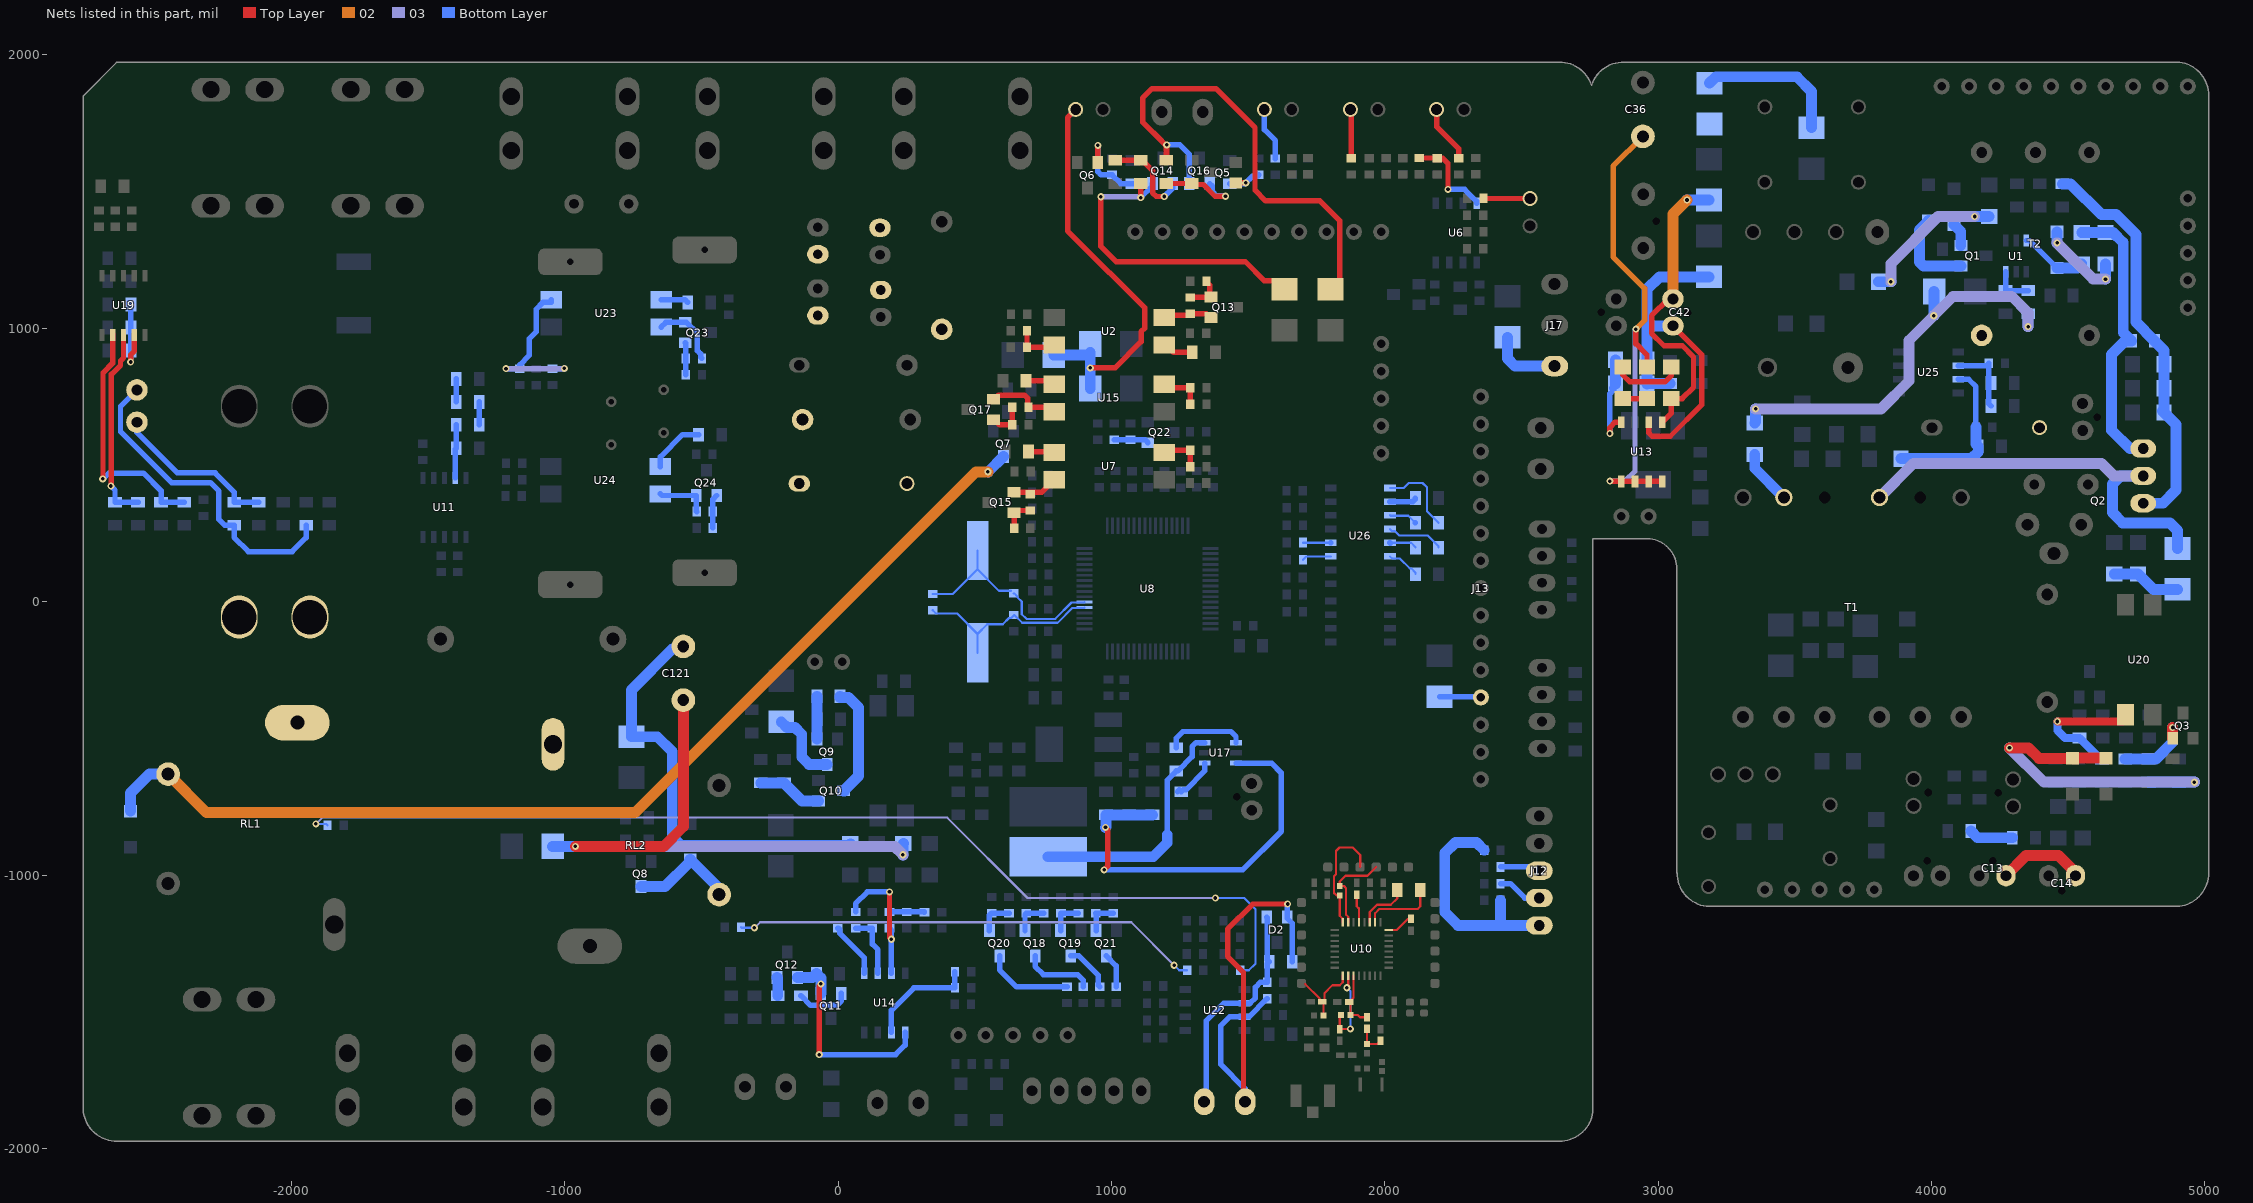
[diagram p0: the nets of this part, all layers, seen from the top]
# Altium PCB MISC105418.PcbDoc (part 5 of 7)
Units mil, origin at the board's own origin, x right, y up, seen from the top; angles counter-clockwise.
Board outline 7774.32 x 3947.04 mil, 4 copper layers (Top Layer, 02, 03, Bottom Layer), stack 30.635 mil thick; 459 components, 285 nets, 1258 pads, 468 vias.
Unrouted connection lines stored in the file: 23.

## Via types
v1: diameter 26, hole 13, Top Layer to Bottom Layer, tented both sides, 468 vias

## Nets (pads, with @x,y where several pads share a name; then routed paths per layer and width w, separated by ;. In a path a pad name is that pad's centre, name@x,y a point inside that pad or via, vN(x,y) a via of type N, cw(c..) or ccw(c..) an arc to the next point about the centre after c; other vN are vias at no path point) (continued)
NetC13_2: C13.2 C14.1 | length 321.8
  Top Layer w40: C13.2@4272.11,-1002.49 4345.61,-929 4464.5,-929 4526.11,-990.61 C14.1@4526.11,-1002.49
NetC17_2: C17.2 U26.2 | length 100.9
  Bottom Layer w20: U26.2@2018.36,365.7 2101.99,365.7 2111.68,375.39 C17.2@2111.68,379
NetC18_1: C18.1 U26.3 | length 106.4
  Bottom Layer w8: U26.3@2018.36,315.7 2020.06,314 2085.8,314 C18.1@2111.68,288.12
  Bottom Layer w20: C18.1@2110.51,289.29 C18.1@2111.68,288.12
NetC18_2: C18.2 U26.1 | length 297.3
  Bottom Layer w8: U26.1@2018.36,415.7 2068.7,415.7 2087,434 2138,434 2154,418 2154,330.44 C18.2@2196.32,288.12
NetC19_1: C19.1 U26.5 | length 95.2
  Bottom Layer w8: U26.5@2027.81,215.7 2095.99,215.7 2111.68,200.02 C19.1@2111.68,197.52
  Bottom Layer w20: U26.5@2018.36,215.7 U26.5@2020.04,214.03
NetC19_2: C19.2 U26.4 | length 209.3
  Bottom Layer w8: U26.4@2018.36,265.7 2026.06,258 2037,258 2053,242 2157.16,242 2196.32,202.83 C19.2@2196.32,197.52
NetC23_2: C23.2 U26.6 | length 123.4
  Bottom Layer w8: U26.6@2018.36,165.7 2026.56,157.5 2054.97,157.5 2090.77,121.7 2096.09,121.7 2111.77,106.02 C23.2@2111.77,100.7
NetC27_1: C27.1 U17.1 | length 293.8
  Bottom Layer w20: C27.1@1237.09,-534.64 1237.09,-498.91 1261,-475 1437,-475 1455.48,-493.48 U17.1@1455.48,-515.6
NetC27_2: C27.2 L29.1 U17.6 | length 902
  Bottom Layer w20: 1204,-853 1204,-652.38 C27.2@1237.09,-619.29 1242.71,-619.29 1295,-567 1295,-530 1309.4,-515.6 U17.6@1340.91,-515.6
  Bottom Layer w39.37: L29.1@768,-933.03 1152.97,-933.03 1204,-882 1204,-853
NetC33_2: C33.2 R36.2 R37.1 U17.3 | length 1481.4
  Top Layer w20: v1(973,-981) 986,-968 986,-834 v1(978,-826)
  Bottom Layer w20: v1(973,-981) 1480,-981 1621,-840 1621,-626 1585.4,-590.4 U17.3@1455.48,-590.4
  Bottom Layer w40: v1(978,-826) 980.08,-823.92 C33.2@980.08,-779.82 R36.2@1065.08,-779.82 R37.1@1150.08,-779.82
NetC36_1: C36.1 D3.2 R92.2 U13.5 U13.6 U13.7 U13.8 | length 1788.1
  Top Layer w19.68: v1(2823,441) 2824.27,439.73 U13.5@2865,439.73 U13.6@2915,439.73 U13.7@2965,439.73 U13.8@3015,439.73 ; v1(2918,997) 2918,944 2959,903 R92.2@2959,857.56
  02 w19.68: v1(2918,997) 2950,1029 2950,1146 2835,1261 2835,1593 C36.1@2944,1702
  03 w19.68: v1(2823,441) 2879,441 2915,477 2915,994 v1(2918,997)
NetC38_2: C38.2 U10.8 | length 99.5
  Top Layer w8: U10.8@2013.52,-1201.6 2042.4,-1201.6 2083.46,-1160.54 C38.2@2096,-1160.54
NetC39_2: C39.2 R44.2 U8.6 Y1.1 | length 777.4
  Bottom Layer w8: R44.2@346,27.72 419.61,27.72 Y1.1@510,118.11 ; Y1.1@510,187.01 Y1.1@510,118.11 ; C39.2@632.28,40 588.11,40 Y1.1@510,118.11 ; C39.2@642,30.28 644.56,30.28 655.72,19.12 655.72,16.56 672,0.28 672,-46 689,-63 794,-63 853.98,-3.02 900.46,-3.02 U8.6@901.78,-1.71
NetC42_1: C42.1 D9.2 R39.1 U13.1 | length 1130
  Top Layer w19.68: U13.1@3015,656.27 3048,689.27 R39.1@3048,742.44 3087.44,742.44 3129,784 3129,895 3088,936 3021,936 2976,981 2976,1046 3037.02,1107.02 C42.1@3053.8,1107.02
  02 w39.37: C42.1@3053.8,1107.02 3053.8,1417.8 v1(3105.2,1469.2)
  Bottom Layer w39.37: v1(3105.2,1469.2) D9.2@3186,1469.2
NetC42_2: C42.2 D4.2 L1.1 R45.1 R88.1 U13.2 | length 1391.7
  Top Layer w19.68: U13.2@2965,656.27 2965,618 2978,605 3044,605 3159,720 3159,904.18 C42.2@3054.2,1008.98
  Bottom Layer w40: L1.1@3042.88,797.79 2960.71,797.79 R88.1@2959.42,796.5 R45.1@2959.42,884.55 2959.42,1017 ; C42.2@3054.2,1008.98 2967.44,1008.98 2959.42,1017 ; D4.2@3186,1188 3004,1188 2959.42,1143.42 2959.42,1017
NetC59_1: C59.1 C63.2 L11.2 | length 108.7
  Top Layer w8: C59.1@1935.09,-1563.03 L11.2@1935.09,-1617.95 1972.63,-1617.95 C63.2@1984.09,-1606.49
NetC59_2: C59.2 C61.2 L21.2 U10.27 | length 216
  Top Layer w8: U10.27@1885.57,-1368.92 1885.57,-1449.02 C61.2@1869.55,-1465.03 1873.97,-1469.45 L21.2@1873.97,-1512.03 1901.03,-1512.03 1909,-1520 1934.98,-1520 C59.2@1935.09,-1520.11
NetC60_2: C60.2 L21.1 U10.26 | length 294.3
  Top Layer w8: L21.1@1839.89,-1512.03 1835.09,-1516.83 C60.2@1835.09,-1563.57 1873.52,-1563.57 v1(1874.09,-1563) ; v1(1861,-1412.5) 1865.88,-1407.61 U10.26@1865.88,-1368.92
  Bottom Layer w8: v1(1861,-1412.5) 1874.09,-1425.59 v1(1874.09,-1563)
NetC79_2: C79.2 C80.1 | length 162.1
  Bottom Layer w40: C80.1@4143.42,-839.18 4167.99,-863.75 C79.2@4295.38,-863.75
NetC82_1: C82.1 Q3.1 R32.1 | length 292.5
  Top Layer w40: Q3.1@4881.69,-499.76 v1(4881.69,-460.31)
  Bottom Layer w40: C82.1@4708.09,-575.85 R32.1@4793.09,-575.85 ; R32.1@4793.09,-575.68 4820.32,-575.68 4881.69,-514.31 v1(4881.69,-460.31)
NetC89_1: C89.1 R181.1 U6.4 | length 338.1
  Top Layer w20: C89.1@2126,1622.91 2190.82,1622.91 R181.1@2192,1621.72 2212.28,1621.72 2231,1603 v1(2231,1508)
  Bottom Layer w20: v1(2231,1508) 2292.08,1508 2336.09,1463.98 U6.4@2336.09,1457.5
NetC98_1: C98.1 R182.2 U19.2 | length 916.8
  Top Layer w20: v1(-2690,449) -2690,451 -2689,452 -2689,837 -2653.37,872.63 U19.2@-2653.37,975.73
  Bottom Layer w20: v1(-2690,449) -2688.38,449 -2667.38,470 -2541,470 -2476.66,405.66 R182.2@-2476.66,363.96 C98.1@-2392.18,363.96
NetC99_2: C99.2 R184.2 U19.3 | length 721.2
  Top Layer w20: v1(-2660,423) -2658,425 -2658,831 -2625,864 -2625,880.64 -2614,891.64 -2614,913.4 U19.3@-2614,975.73
  Bottom Layer w20: v1(-2660,423) -2645.15,408.15 R184.2@-2645.15,363.96 C99.2@-2560.91,363.96
NetC100_1: C100.1 R187.1 R188.1 U19.4 | length 315.6
  Top Layer w20: v1(-2588,876.62) -2588,902.63 -2574.63,916 U19.4@-2574.63,975.73
  Bottom Layer w20: v1(-2588,876.62) -2586.91,877.72 R187.1@-2586.91,918.67 C100.1@-2586.91,1002.7 R188.1@-2586.91,1087.17
NetC101_1: C101.1 U10.13 | length 104
  Top Layer w8: C101.1@1897,-1071.49 1897,-1114 1905.25,-1122.25 U10.13@1905.25,-1172.07
NetC110_1: C110.1 R44.1 U8.5 Y1.2 | length 724.1
  Bottom Layer w8: R44.1@346,-31.72 357.16,-42.88 434.77,-42.88 Y1.2@510,-118.11 ; Y1.2@510,-187.01 Y1.2@510,-118.11 ; U8.5@901.84,-21.45 900.58,-22.71 857.29,-22.71 803,-77 673.01,-77 644.56,-48.55 633.4,-59.71 625.29,-59.71 602.26,-82.74 545.37,-82.74 Y1.2@510,-118.11
NetC114_1: C114.1 R81.1 R82.2 | length 127.9
  Bottom Layer w20: R81.1@188.3,-1134.98 R82.2@251.44,-1134.98 314.57,-1134.98 C114.1@315.76,-1136.16
NetC119_1: C119.1 R193.1 R194.2 U25.2 | length 275.2
  Bottom Layer w19.68: U25.2@4097.36,863.5 4200.55,863.5 C119.1@4209.05,872 4209.05,724.05 R194.2@4217.57,715.53
NetC120_2: C120.2 R191.1 R192.2 U25.3 | length 610.6
  Bottom Layer w19.68: U25.3@4097.36,813.5 4135.5,813.5 4162.05,786.95 C120.2@4162.05,638.5
  Bottom Layer w40: R191.1@3888.56,523.35 4146.35,523.35 4170.57,547.57 R192.2@4170.57,568.5 4162.05,577.03 C120.2@4162.05,638.5
NetC121_1: C121.1 D29.2 R263.2 | length 2235.2
  Top Layer w40: v1(-961,-895) -638,-895 -566.28,-823.28 -566.28,-500.28 C121.1@-566.28,-360.31
  03 w40: v1(-961,-895) 206,-895 v1(237,-926)
  Bottom Layer w40: D29.2@-1044.2,-895 v1(-961,-895) ; C121.1@-566.28,-360.31 C121.1@-566.28,-347.7 ; v1(237,-926) 237,-886.87 R263.2@238.43,-885.44
NetC121_2: C121.2 D30.1 R200.2 | length 1577.5
  Bottom Layer w39.37: C121.2@-566.28,-163.47 -575.32,-172.5 -605.5,-172.5 -756,-323 D30.1@-756,-493.77 -661.23,-493.77 -607,-548 -607,-859 -574,-892 38.54,-892 R200.2@45.09,-885.44
NetC129_1: C129.1 R42.2 U10.25 | length 283.8
  Top Layer w8: 1709,-1399 1761,-1451 1761,-1453.4 C129.1@1771.17,-1463.58 ; R42.2@1775.59,-1513.58 1775.59,-1467.99 C129.1@1771.17,-1463.58 ; U10.25@1846.2,-1368.92 1846.2,-1392.02 1835.22,-1403 1808,-1403 1779,-1432 1779,-1455.75 C129.1@1771.17,-1463.58
NetCX1_1: CX1.1 L28.2 L30.1 Y2.1
NetCX1_2: CX1.2 L26.2 L27.1 Y3.2
NetCX3_1: CX3.1 T2.4
NetD2_1: D2.1 J7.1 R176.1 R178.2 U22.6 | length 847.9
  Bottom Layer w19.68: D2.1@1567.8,-1154.24 1569.67,-1156.11 1569.67,-1310.15 R176.1@1576.65,-1317.14
  Bottom Layer w20: J7.1@1338.98,-1829.5 1346.45,-1822.02 1346.45,-1533.55 1411.04,-1468.96 U22.6@1486.06,-1468.96 1507.04,-1468.96 1526,-1450 1526,-1411 1544.86,-1392.14 R178.2@1569.31,-1392.14 1569.31,-1324.48 R176.1@1576.65,-1317.14
NetD2_2: D2.2 J7.2 R171.1 R176.2 U22.7 | length 1661
  Top Layer w19.68: J7.2@1488.98,-1829.5 1483,-1823.52 1483,-1356 1425,-1298 1425,-1198 1517,-1106 v1(1644,-1106)
  Bottom Layer w19.68: v1(1644,-1106) 1642.6,-1107.4 D2.2@1642.6,-1154.24 1642.6,-1158.17 1661.3,-1176.87 R176.2@1661.3,-1317.14
  Bottom Layer w20: J7.2@1488.98,-1829.5 1488.98,-1781.98 1399,-1692 1399,-1552 1432.04,-1518.96 U22.7@1486.06,-1518.96 1502.49,-1518.96 R171.1@1569.31,-1452.14
NetD3_1: D3.1 D11.2 | length 537.1
  Bottom Layer w40: D3.1@3188,1896.8 3211.2,1920 3506.8,1920 3561,1865.8 D11.2@3561,1733.8
NetD6_2: D6.2 D10.2 D19.2 J25.2 | length 1480
  Top Layer w20: J25.2@869.09,1800.5 839.17,1770.58 839.17,1356.54 993.56,1202.16 994.84,1202.16 1122,1075 1122,1000.77 1108.78,987.55 1108.78,950.78 1013,855 v1(922.2,855)
  Bottom Layer w40: D19.2@788.8,901.67 912.86,901.67 922.2,911 v1(922.2,855) D10.2@922.2,780
NetD7_2: D7.2 J17.1 | length 262.3
  Bottom Layer w40: D7.2@2448.09,966.9 2448.09,888.91 2475.3,861.7 J17.1@2621.09,861.7
NetD8_2: D8.2 Q14.2 R129.1 | length 1186.6
  Top Layer w19.68: v1(961,1481) 961,1299.71 1017,1243.71 1489.29,1243.71 1558.7,1174.3 1601.5,1174.3 D8.2@1633,1142.8 ; v1(1107,1478) 1107.13,1478.13 1107.13,1529.55 R129.1@1107.26,1529.68
  03 w19.68: v1(961,1481) 1104,1481 v1(1107,1478)
  Bottom Layer w19.68: v1(1107,1478) 1149.69,1520.69 Q14.2@1149.69,1529.62
NetD12_1: D12.1 Q7.3 RL1.2 | length 3885.7
  02 w40: RL1.2@-2450.87,-631 -2309.87,-772 -743,-772 504,475 v1(548,475)
  Bottom Layer w40: D12.1@-2588,-766.06 -2588,-700 -2519,-631 RL1.2@-2450.87,-631 ; v1(548,475) 549.26,475 Q7.3@605,530.74
NetD13_1: D13.1 Q8.3 RL2.2 | length 393.9
  Bottom Layer w40: Q8.3@-721.34,-1042.41 -633.41,-1042.41 -544.62,-953.62 -544.62,-946.58 -541.98,-943.94 D13.1@-540.02,-943.94 ; D13.1@-537.38,-946.58 -444.13,-1039.83 -444.13,-1063.03 RL2.2@-435.21,-1071.94
NetD14_1: D14.1 Q9.3 | length 281.1
  Bottom Layer w40: D14.1@-207.91,-439.47 -186.57,-460.81 -157.19,-460.81 -133,-485 -133,-568 -105.74,-595.26 Q9.3@-40,-595.26
NetD16_2: D16.2 Q16.2 R135.1 | length 1862.1
  Top Layer w20: v1@1199.57,1668.57 1200.26,1667.87 R135.1@1200.26,1614.32 1202,1616.06 v1(1202,1671) 1197.13,1671 1171.07,1697.06 1130.07,1738.07 1114,1754.13 1114,1842 1149,1877 1382.28,1877 1525,1734.28 1525,1505 1564,1466 1762,1466 1835,1393 1835,1174.14 1803.66,1142.8 D16.2@1801,1142.8
  Bottom Layer w20: v1(1202,1671) 1250,1671 1284.69,1636.31 Q16.2@1284.69,1529.62
NetD20_1: D20.1 Q1.2 | length 85.9
  Bottom Layer w39.37: D20.1@4082.09,1378.54 4106.83,1353.8 Q1.2@4106.83,1302.91
NetD21_1: D21.1 R12.1 | length 327.8
  03 w40: v1(4459.09,1312.09) 4591.09,1180.09 v1(4636.09,1180.09)
  Bottom Layer w40: v1@4459,1312 v1(4459.09,1312.09) D21.1@4459.09,1352.39 ; v1(4636.09,1180.09) R12.1@4636.09,1235.78
NetD21_2: D21.2 R10.1 U1.6 | length 250.7
  Bottom Layer w19.68: U1.6@4346.4,1321.09 4358.51,1321.09 D21.2@4459.09,1220.5
  Bottom Layer w39.37: D21.2@4459.09,1220.5 4533.82,1220.5 R10.1@4549.09,1235.78
NetD22_1: D22.1 R6.1 R20.1 | length 1519.1
  03 w40: v1(3356,705) 3815,705 3918,808 3918,956 v1(4008,1046) 4079,1117 4293,1117 4353,1057 v1(4353,1006)
  Bottom Layer w40: R20.1@3353,653.56 3356,656.56 v1(3356,705) ; v1(4008,1046) 4009.29,1047.29 D22.1@4009.29,1134.5 ; v1(4353,1006) 4353.09,1006.09 R6.1@4353.09,1053.18
NetD23_1: D23.1 Q2.2 T1.3 | length 1595.7
  03 w40: T1.3@3809.09,381.08 3933.02,505 4622,505 4667.03,459.97 Q2.2@4773.87,459.97
  Bottom Layer w40: Q2.2@4773.87,459.97 4690.97,459.97 4661,430 4661,326 4699,288 4872,288 4899.09,260.91 D23.1@4899.09,194.31
NetD23_2: D23.2 R17.1 R19.1 | length 254.5
  Bottom Layer w40: R17.1@4668.09,101.32 R19.1@4755.09,101.32 4811.71,44.7 D23.2@4899.09,44.7
NetD555_2: D555.2 J13.12 | length 151.9
  Bottom Layer w20: D555.2@2200.09,-348.1 2348.9,-348.1 J13.12@2351.09,-350.3
NetJ1_2: J1.2 R113.2 | length 212.3
  Top Layer w20: J1.2@2189.09,1800.5 2189.09,1737.91 2270,1657 R113.2@2270,1621.72
NetJ2_2: J2.2 R114.2 | length 170.5
  Top Layer w20: R114.2@2361.09,1476 2362.39,1474.7 J2.2@2531.09,1474.7
NetJ3_2: J3.2 R121.1 | length 180
  Top Layer w20: J3.2@1874.09,1800.5 1877,1797.6 R121.1@1877,1621.72
NetJ4_2: J4.2 R122.1 | length 196.4
  Bottom Layer w20: J4.2@1559.09,1800.5 1559.09,1726.91 1599.09,1686.91 R122.1@1599.09,1620.69
NetJ12_1: J12.1 R233.2 R234.1 | length 848.4
  Bottom Layer w40: R233.2@2363.65,-909.5 2335.15,-881 2258,-881 2219,-920 2219,-1135 2268.3,-1184.3 2559.09,-1184.3 J12.1@2565.09,-1190.3 ; 2423.09,-1184.3 R234.1@2423.09,-1092.5
NetJ12_2: J12.2 R235.1 | length 163.9
  Bottom Layer w20: R235.1@2423.09,-1031.5 2459.5,-1031.5 2512.3,-1084.3 J12.2@2565.09,-1084.3
NetJ12_3: J12.3 R236.1 | length 147.7
  Bottom Layer w20: R236.1@2423.09,-970.5 2551.29,-970.5 J12.3@2565.09,-984.3
NetJP1_2: pad.1@-2191,-56.5 RL1.1
NetJP2_2: pad.1@-1932,-56.5 RL2.4
NetL22_1: L22.1 U10.10 | length 267.6
  Top Layer w8: U10.10@1964.31,-1172.07 1964.31,-1139.69 1980,-1124 2120,-1124 2129.65,-1114.35 L22.1@2129.65,-1055
NetL22_2: L22.2 U10.11 | length 188.5
  Top Layer w8: U10.11@1944.62,-1172.07 1944.62,-1135.38 1971,-1109 2022,-1109 2045,-1086 L22.2@2045,-1055
NetQ1_1: Q1.1 R11.2 ZD1.2 | length 322.2
  Bottom Layer w40: ZD1.2@3989.09,1393.5 3955.57,1359.98 R11.2@3955.57,1289.13 3955.57,1242.43 3969.9,1228.1 Q1.1@4106.83,1228.1
NetQ2_1: Q2.1 R10.2 R12.2 R15.1 | length 1053.4
  Bottom Layer w40: R10.2@4549.09,1350.9 R12.2@4636.09,1350.9 4663.1,1350.9 4701,1313 4701,983.99 R15.1@4730.99,954 4708,954 4658,904 4658,627 4725.03,559.97 Q2.1@4773.87,559.97
NetQ2_3: Q2.3 R9.2 R13.1 R15.2 R16.1 R241.1 | length 1489
  Bottom Layer w40: R9.2@4478.09,1528.35 4508.65,1528.35 4621,1416 4674,1416 4747,1343 4747,1022.64 R15.2@4815.64,954 4850.56,919.08 R16.1@4850.56,869 R13.1@4850.56,780.5 R241.1@4850.56,692 ; Q2.3@4773.87,359.97 4845.97,359.97 4894,408 4894,648.56 R241.1@4850.56,692 ; R241.1@4845.34,697.22 R241.1@4850.56,692
NetQ5_1: Q5.1 R56.2 R58.2 | length 152.5
  Top Layer w20: Q5.1@1454.52,1531.6 1454.72,1531.8 1490.8,1531.8 v1(1491,1532)
  Bottom Layer w20: R58.2@1432.09,1528.7 v1@1487.7,1528.7 ; v1(1491,1532) 1515.08,1556.08 1533.94,1556.08 R56.2@1539.09,1561.24
NetQ6_1: Q6.1 R57.1 R59.2 | length 304.4
  Top Layer w20: Q6.1@949.66,1606.34 949.83,1606.51 949.83,1668.83 v1(950,1669)
  Bottom Layer w20: v1(950,1669) 949.83,1668.83 949.83,1573.12 961.72,1561.24 R57.1@1002.09,1561.24 1034.63,1528.7 R59.2@1077.09,1528.7
NetQ9_1: Q9.1 R69.2 R70.2 | length 156.8
  Bottom Layer w40: Q9.1@-77.4,-502.74 Q9.1@-77.4,-502.74 -77.36,-346.04 R69.2@-77.32,-346
NetQ10_1: Q10.1 R72.2 R73.2 | length 238
  Bottom Layer w40: R73.2@-282.91,-663.44 -197.91,-663.44 -131.94,-729.4 Q10.1@-72.26,-729.4
NetQ10_3: Q10.3 R69.1 | length 416.6
  Bottom Layer w40: R69.1@7.32,-346 7.32,-350.69 7.64,-351 38.25,-351 75,-387.75 75,-637.26 23.88,-688.38 23.88,-691.69 23.57,-692 Q10.3@20.26,-692
NetQ11_1: Q11.1 Q12.1 R75.2 U14.1 | length 789.6
  Top Layer w20: v1(-69,-1657) -69,-1405.54 -63.31,-1399.84 v1(-63.31,-1398.22)
  Bottom Layer w20: v1(-69,-1657) 210.55,-1657 245.09,-1622.46 U14.1@245.09,-1575.76
  Bottom Layer w40: Q12.1@-148.5,-1374.54 -93.04,-1374.54 R75.2@-79.32,-1360.82 -63.31,-1376.83 v1(-63.31,-1398.22) Q11.1@-63.31,-1432.7
NetQ11_2: Q11.2 R97.1 | length 196.7
  Bottom Layer w20: R97.1@-135.91,-1441.5 -100.4,-1477 -5,-1477 11.5,-1460.5 Q11.2@11.5,-1432.7
NetQ12_2: Q12.2 R99.2 | length 68
  Bottom Layer w40: Q12.2@-223.31,-1374.54 -220.91,-1376.94 R99.2@-220.91,-1441.5
NetQ13_1: Q13.1 R64.1 R65.2 | length 140.7
  Top Layer w20: R64.1@1288.58,1112.79 1289.34,1113.55 1363.47,1113.55 Q13.1@1364.23,1114.31 1360.29,1118.24 1360.29,1156.89 1347.83,1169.35 R65.2@1347.83,1171.91
NetQ13_2: Q13.2 R64.2 U2.2 | length 183.1
  Top Layer w20: U2.2@1192.79,1038.91 1202.07,1048.18 1283.42,1048.18 R64.2@1288.58,1053.34 1346.45,1053.34 1360.29,1039.5 Q13.2@1364.23,1039.5
NetQ14_1: Q14.1 R129.2 R130.2 | length 341.6
  Top Layer w20: R130.2@1014.26,1614.32 1112.57,1614.32 1150.54,1576.35 1150.54,1495.46 1164,1482 v1(1193,1482)
  Bottom Layer w20: v1(1193,1482) 1224.5,1513.5 Q14.1@1224.5,1529.62
NetQ15_1: Q15.1 R80.1 R85.1 | length 120
  Top Layer w19.68: R85.1@643.89,268 Q15.1@643.89,325.6 651.57,333.28 R80.1@703.15,333.28
NetQ15_2: Q15.2 R80.2 U7.2 | length 177.1
  Top Layer w19.68: Q15.2@643.89,400.4 R80.2@695.47,400.4 ; R80.2@703.15,392.72 R80.2@695.47,400.4 ; U7.2@791.21,446 745.61,400.4 R80.2@695.47,400.4
NetQ16_1: Q16.1 R135.2 R136.2 | length 324.7
  Top Layer w19.68: R135.2@1200.26,1529.68 R136.2@1293.26,1529.7 1297.21,1525.74 1336.26,1525.74 1379,1483 v1(1417,1483)
  Bottom Layer w19.68: Q16.1@1359.5,1529.62 1369.34,1519.78 1369.34,1499.66 1384.79,1484.21 1415.79,1484.21 v1(1417,1483)
NetQ17_1: Q17.1 R90.1 R91.1 | length 151.8
  Top Layer w19.68: Q17.1@571.9,669.1 Q17.1@568,665.2 571.94,665.2 590.13,647 R91.1@637.28,647 R90.1@637.28,711 R90.1@633.37,707.1
NetQ17_2: Q17.2 R90.2 U15.2 | length 272.1
  Top Layer w20: Q17.2@568,740 571.94,740 587.3,755.37 682.28,755.37 694,743.65 694,713.72 R90.2@696.72,711 775.21,711 U15.2@791.21,695
NetQ18_1: Q18.1 R47.1 R49.1 | length 129.3
  Bottom Layer w20: Q18.1@683.58,-1203.24 683.58,-1144.55 R49.1@688.63,-1139.5 R47.1@752.1,-1139.5
NetQ18_3: Q18.3 R213.2 | length 259.1
  Bottom Layer w20: Q18.3@720.98,-1295.76 720.98,-1333.98 751,-1364 876,-1364 897.25,-1385.25 R213.2@897.25,-1408.62
NetQ19_1: Q19.1 R48.1 R50.1 | length 128
  Bottom Layer w20: Q19.1@813.58,-1203.24 813.58,-1141.49 R50.1@815.57,-1139.5 R48.1@879.04,-1139.5
NetQ19_3: Q19.3 R214.2 | length 174.6
  Bottom Layer w20: Q19.3@850.98,-1295.76 880.76,-1295.76 951,-1366 951,-1402.64 R214.2@957.25,-1408.9
NetQ20_1: Q20.1 R51.1 R52.1 | length 130.6
  Bottom Layer w20: Q20.1@553.58,-1203.24 553.58,-1147.61 R52.1@561.69,-1139.5 R51.1@625.16,-1139.5
NetQ20_3: Q20.3 R125.2 | length 323.3
  Bottom Layer w20: Q20.3@590.98,-1295.76 590.98,-1346.98 652.9,-1408.9 R125.2@837.45,-1408.9
NetQ21_1: Q21.1 R127.1 R128.1 | length 127.7
  Bottom Layer w20: Q21.1@943.58,-1203.24 943.58,-1140.56 R128.1@942.51,-1139.5 R127.1@1005.98,-1139.5
NetQ21_3: Q21.3 R126.2 | length 128.2
  Bottom Layer w20: Q21.3@980.98,-1295.76 1017.25,-1332.03 R126.2@1017.25,-1408.9
NetQ22_1: Q22.1 R238.1 R239.1 | length 127.5
  Bottom Layer w20: R238.1@1009.7,592.28 R239.1@1069.36,592.28 1122.06,592.28 Q22.1@1132.74,581.6
NetQ23_1: Q23.1 R108.1 R109.2 | length 118.2
  Bottom Layer w20: Q23.1@-559.02,947.1 -557.57,945.65 R108.1@-557.57,889.5 R109.2@-557.57,829.5
NetQ23_2: Q23.2 R108.2 U23.2 | length 255.9
  Bottom Layer w20: U23.2@-647.73,1004.5 -630.33,1021.91 -555.09,1021.91 -515,981.82 -515,917.81 -503.28,906.09 -503.28,894.66 R108.2@-498.12,889.5
NetQ24_1: Q24.1 R111.1 R112.1 | length 124.5
  Bottom Layer w20: R112.1@-458.12,269.5 R111.1@-458.12,329.5 -458.12,374.41 Q24.1@-444.28,388.24
NetQ24_2: Q24.2 R111.2 U24.2 | length 191.8
  Bottom Layer w20: U24.2@-650.12,394.12 -644.24,388.24 Q24.2@-519.09,388.24 ; Q24.2@-518.33,387.49 -518.33,330.26 R111.2@-517.57,329.5
NetR5_2: R5.2 R8.1 | length 542.7
  03 w39.37: v1(3851,1170) 3851,1236 4023.78,1408.78 v1(4157,1408.78)
  Bottom Layer w39.37: R5.2@3805,1170 v1(3851,1170) ; v1(4157,1408.78) R8.1@4210.09,1408.78
NetR6_2: R6.2 R7.1 U1.3 | length 152.3
  Bottom Layer w19.68: U1.3@4271.6,1206.52 4271.6,1139.31 R7.1@4270.09,1137.81 R6.2@4353.09,1137.83
NetR18_2: R18.2 U26.12 | length 101.8
  Bottom Layer w8: R18.2@1700.82,216.43 1701.55,215.7 U26.12@1801.83,215.7
  Bottom Layer w20: U26.12@1801.46,216.07 U26.12@1801.83,215.7
NetR20_2: R20.2 T1.5 | length 201.5
  Bottom Layer w39.37: R20.2@3353,538.44 3353,487.57 T1.5@3459.49,381.08
NetR21_1: R21.1 R25.2 U20.1 | length 507.1
  Top Layer w30: v1(4460,-438.51) 4698.49,-438.51 4709.09,-427.91 U20.1@4709.09,-413.28
  Bottom Layer w30: v1(4460,-438.51) 4460,-471 4488.14,-499.14 R21.1@4541.09,-499.14 4617.8,-575.85 R25.2@4623.09,-575.85
NetR32_2: R32.2 R33.1 ZD2.1 ZD3.1 | length 1264.9
  Top Layer w40: v1(4285,-535) 4354.95,-535 4392.95,-573 4514.7,-573 ZD3.1@4515.09,-572.61 ZD2.1@4638.09,-572.61
  03 w40: v1(4285,-535) 4410.5,-660.5 v1(4961,-660.5)
  Bottom Layer w40: R32.2@4793.09,-660.5 v1(4961,-660.5)
NetR35_2: R35.2 U17.4 | length 155.7
  Bottom Layer w20: R35.2@1241.41,-695.17 R35.2@1248.25,-688.33 ; R35.2@1255.09,-695.17 1262,-688.27 1271.73,-688.27 1340.91,-619.09 U17.4@1340.91,-590.4
NetR38_1: R38.1 R39.2 | length 255.8
  Top Layer w19.68: R38.1@2870,857.56 2870,830 2896,804 3024,804 3048,828 R39.2@3048,857.56
NetR38_2: R38.2 R92.1 | length 89
  Top Layer w19.68: R38.2@2870,742.44 R92.1@2959,742.44
NetR40_1: R40.1 R61.1 U2.4 | length 163.7
  Top Layer w20: R61.1@690.89,990.81 R40.1@690.89,930.81 783.12,930.81 U2.4@791.21,938.91
NetR43_1: R43.1 U10.15 | length 325.1
  Top Layer w8: U10.15@1865.88,-1172.07 1865.88,-1153 1858,-1145.12 1858,-1048 1850.37,-1040.37 R43.1@1835.09,-1040.37 1835.09,-1023.91 1856,-1003 1936.3,-1003 1968.35,-970.94
NetR43_2: R43.2 U10.16 | length 433.4
  Top Layer w8: U10.16@1846.2,-1172.07 1846.2,-1160.1 1835.09,-1149 R43.2@1835.09,-1074.45 1822.91,-1074.45 1814,-1065.54 1814,-1004 1821,-997 1821,-912 1834,-899 1882,-899 1910,-927 1910,-970.94
NetR45_2: R45.2 R88.2 U13.4 | length 356.7
  Top Layer w20: v1(2823,615) 2823,637 2842.27,656.27 U13.4@2865,656.27
  Bottom Layer w20: v1(2823,615) 2823,760 2836.6,773.6 2829,781.2 R88.2@2844.31,796.5
  Bottom Layer w40: R88.2@2844.31,796.5 R45.2@2844.31,884.55
NetR60_1: R60.1 U14.5 | length 206.1
  Bottom Layer w20: R60.1@-1.11,-1194.43 1.45,-1194.43 6.61,-1199.59 6.61,-1213.61 95.09,-1302.09 U14.5@95.09,-1359.23
NetR63_1: R63.1 U2.1 | length 114.1
  Top Layer w20: U2.1@1192.79,938.91 1200.66,938.91 1227.66,911.91 R63.1@1295.73,911.91
NetR66_2: R66.2 U7.1 | length 96.5
  Top Layer w19.68: R66.2@696,549 788.21,549 U7.1@791.21,546
NetR77_1: R77.1 R79.2 U14.2 | length 406.4
  Bottom Layer w20: U14.2@195.09,-1575.76 195.09,-1494.91 277.5,-1412.5 R79.2@427.49,-1412.5 R77.1@427.49,-1353.53
NetR78_1: R78.1 R81.2 U14.7 | length 516.2
  Top Layer w20: v1(188,-1062) 188,-1225.91 190,-1227.91 189,-1228.91 v1(195.09,-1235)
  Bottom Layer w20: R78.1@64,-1134.98 64,-1105 107,-1062 v1(188,-1062) ; R81.2@188.3,-1194.43 195.09,-1201.22 v1(195.09,-1235) U14.7@195.09,-1359.23
NetR78_2: R78.2 R84.2 U14.6 | length 234.4
  Bottom Layer w20: R78.2@64,-1194.43 R84.2@125.17,-1194.43 125,-1194.6 125,-1253 145.09,-1273.09 U14.6@145.09,-1359.23
NetR83_2: R83.2 U26.11 | length 106.3
  Bottom Layer w8: R83.2@1700.82,152.95 1713.57,165.7 U26.11@1801.83,165.7
NetR86_1: R86.1 R87.2 U7.4 | length 159.7
  Top Layer w20: U7.4@1192.79,546 1199.79,553 1286.82,553 R87.2@1288.38,551.44 ; R86.1@1288.38,493.41 R87.2@1288.38,551.44 ; R87.2@1288.38,554 R87.2@1288.38,551.44
NetR89_2: R89.2 U15.1 | length 109.3
  Top Layer w19.68: R89.2@687.38,808.3 777.91,808.3 U15.1@791.21,795
NetR93_2: R93.2 R163.1 U15.4 | length 160.9
  Top Layer w20: U15.4@1192.79,795 1205.88,781.91 R163.1@1288.38,781.91 R93.2@1288.38,722
NetR94_1: R94.1 R102.2 | length 84
  Bottom Layer w20: R102.2@-1312.47,646.5 R94.1@-1312.47,730.52
NetR94_2: R94.2 R231.1 | length 84
  Bottom Layer w20: R94.2@-1397.12,730.52 R231.1@-1397.12,814.53
NetR102_1: R102.1 R232.1 U11.4 | length 190.5
  Bottom Layer w20: U11.4@-1400.54,452.77 -1400.38,452.93 R232.1@-1400.38,558.24 ; R232.1@-1397.12,561.5 R102.1@-1397.12,646.5
NetR104_1: R104.1 R105.1 U23.4 | length 624.4
  03 w20: v1(-1214.8,852.2) -1214.4,852.6 -1001.99,852.6 v1(-1001.59,853)
  Bottom Layer w20: v1(-1214.8,852.2) R105.1@-1164.5,852.2 -1164.5,866.5 -1130.5,900.5 -1130.5,961 -1104.68,986.82 -1104.68,1069.32 -1078.8,1095.2 -1049.31,1095.2 U23.4@-1049.31,1104.5 ; R104.1@-1044.5,852.2 -1044.11,852.6 -1001.99,852.6 v1(-1001.59,853)
NetR107_1: R107.1 U23.1 | length 101.6
  Bottom Layer w20: U23.1@-647.73,1104.5 -560.23,1104.5 R107.1@-550.23,1094.5
NetR110_2: R110.2 U24.1 | length 209.2
  Bottom Layer w20: U24.1@-650.12,494.12 -650.12,529.88 -569.24,610.76 R110.2@-510.23,610.76
NetR117_2: R117.2 RNTC1.1 | length 1713.8
  03 w8: v1(-306,-1193) -305.31,-1193 -285.31,-1173 1072,-1173 v1(1229,-1330)
  Bottom Layer w8: RNTC1.1@-355.28,-1191 -353.28,-1193 v1(-306,-1193) ; v1(1229,-1330) 1247.62,-1348.62 R117.2@1276.63,-1348.62
NetR120_2: R120.2 RNTC2.1 | length 3895.2
  03 w8: v1(-1910,-813) -1887,-790 399,-790 693,-1084 v1(1380,-1084)
  Bottom Layer w8: v1(-1910,-813) -1872.72,-813 RNTC2.1@-1867.72,-818 ; v1(1380,-1084) 1486,-1084 1527,-1125 1527,-1324 1502.38,-1348.62 R120.2@1470.63,-1348.62
NetR123_2: R123.2 R124.1 U12.1 | length 1190.9
  Bottom Layer w20: U12.1@-2564.91,774.5 -2625,714.41 -2625,622 -2438.23,435.23 -2296.23,435.23 -2265,404 -2265,301 -2243.32,279.31 R124.1@-2209,279.31 -2209,235 -2157,183 -1997,183 -1946.14,233.86 R123.2@-1946.14,279.31
NetR124_2: R124.2 R145.2 U12.2 | length 610
  Bottom Layer w20: U12.2@-2564.91,656.39 -2564.91,618.91 -2417,471 -2279,471 -2209,401 R124.2@-2209,363.96 R145.2@-2119.69,363.96